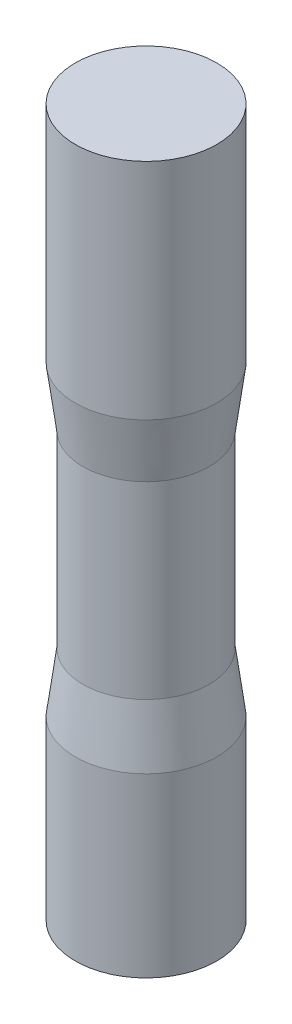
from build123d import *


with BuildPart() as part:
    # Sketch1 → Revolve1 (revolve)
    with BuildSketch(Plane.XY, mode=Mode.PRIVATE) as revolve1_sk:
        Polygon((0, 0), (-3, 0), (-3, -9.5), (-2.675, -12), (-2.675, -20), (-3, -22.5), (-3, -30), (0, -30), align=None)
    revolve(revolve1_sk.sketch.rotate(Axis((0, -30, 0), (0, 1, 0)), 270), axis=Axis((0, -30, 0), (0, 1, 0)))


solid = part.part
